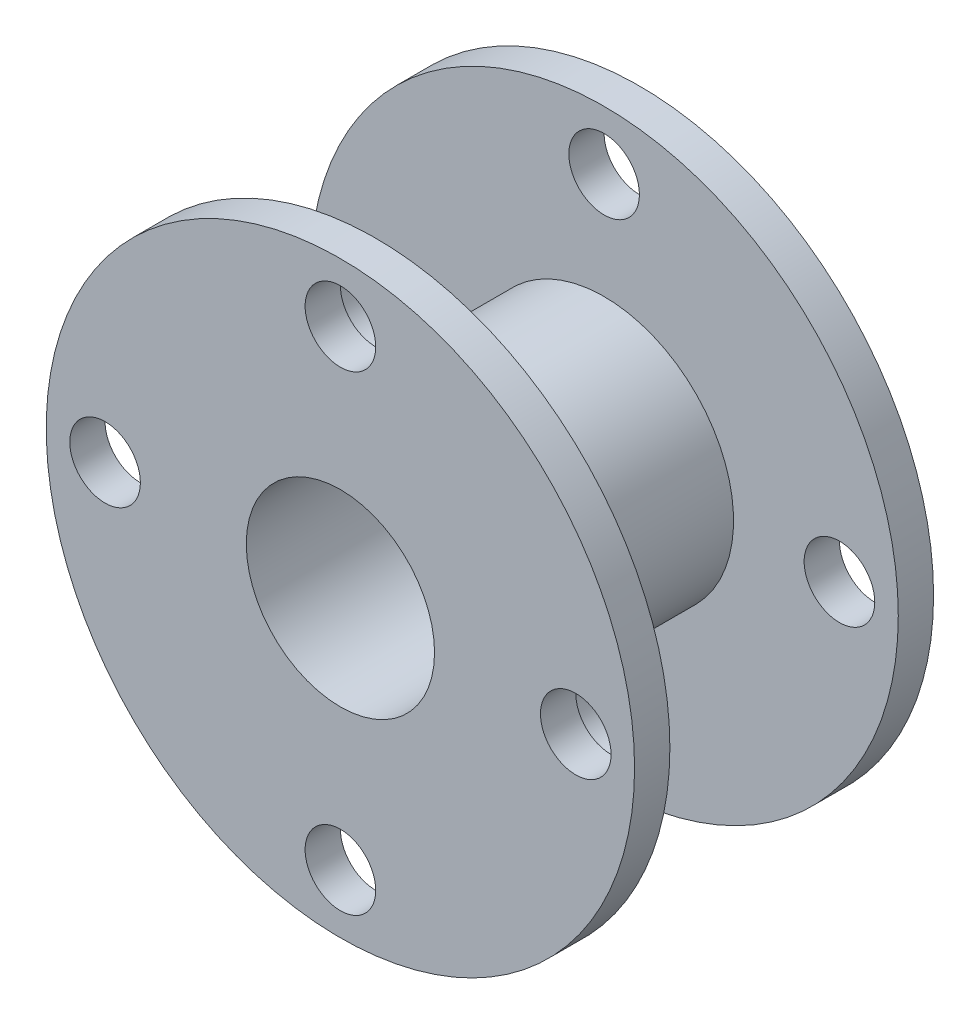
SolidWorks part; units mm, degrees
material "Q235-A"
ref_plane "前视基准面" through (0, 0, 0) normal (0, 0, 1) x (1, 0, 0)
ref_plane "上视基准面" through (0, 0, 0) normal (0, 1, 0) x (1, 0, 0)
ref_plane "右视基准面" through (0, 0, 0) normal (1, 0, 0) x (0, 0, -1)
sketch "草图1" plane through (0, 0, 0) normal (0, 0, 1) x (1, 0, 0)
  circle A0 centre (0, 0) radius 8
  circle A1 centre (0, 0) radius 25 construction
  dimension "D1" = 16
  dimension "D2" = 50
extrude "拉伸-薄壁1" add sketch "草图1" along normal mid plane 25.41 thin
sketch "草图2" plane through (0, 0, 12.705) normal (0, 0, 1) x (1, 0, 0)
  circle A0 centre (0, 0) radius 8 construction
  circle A1 centre (0, 0) radius 8
  circle A2 centre (0, 0) radius 25
  circle A3 centre (0, 20) radius 3
  circle A4 centre (20, 0) radius 3
  circle A5 centre (0, -20) radius 3
  circle A6 centre (-20, 0) radius 3
  point P14 (0, 0)
  dimension "D1" = 50
  dimension "D2" = 6
  dimension "D4" = 40
  dimension "D3" = 4
extrude "凸台-拉伸1" add sketch "草图2" against normal blind 3
mirror "镜向1" about plane through (0, 0, 0) normal (0, 0, 1) of "凸台-拉伸1"
